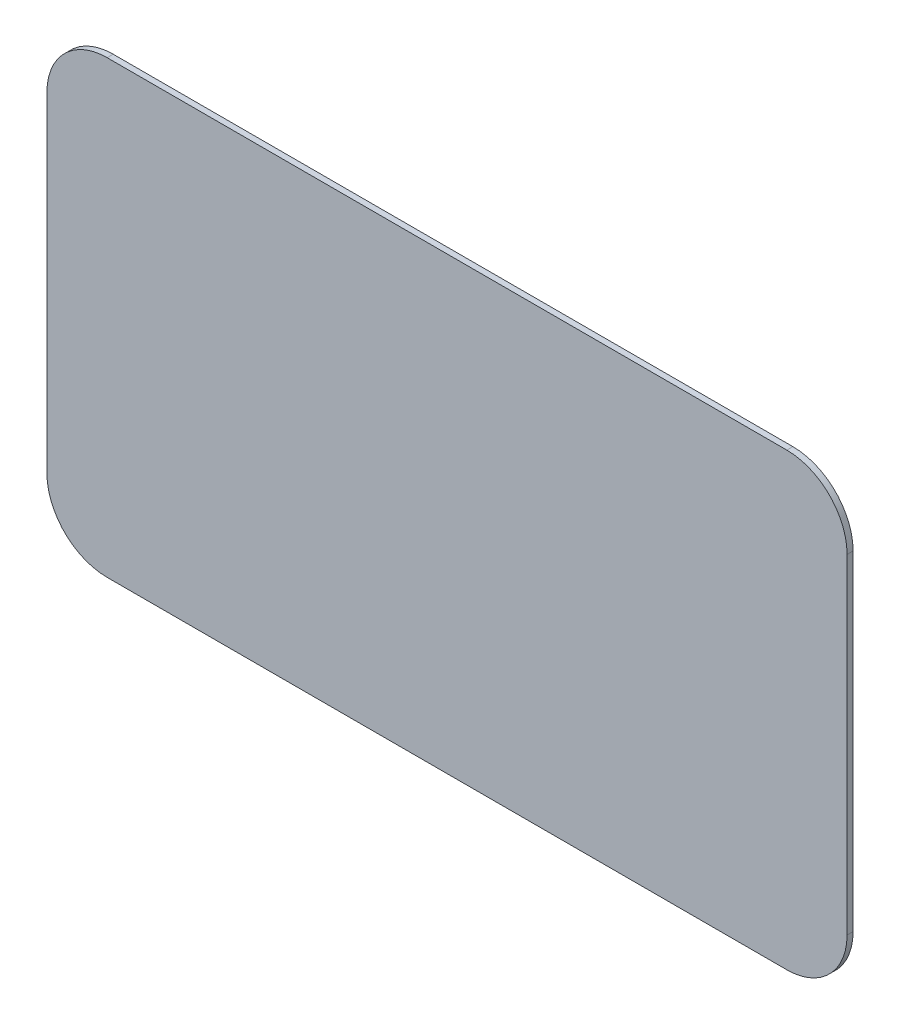
from build123d import *

# Parameters (mm, degrees)
SKETCH1_W           = 132.8
SKETCH1_H           = 74.7
BOSS_EXTRUDE1_DEPTH = 1
FILLET1_R           = 10


with BuildPart() as part:
    # Sketch1 → Boss-Extrude1 (new body)
    with BuildSketch(Plane.XY):
        Rectangle(SKETCH1_W, SKETCH1_H)
    extrude(amount=BOSS_EXTRUDE1_DEPTH)

    # Fillet1
    fillet1_edges = [part.edges().sort_by_distance(p)[0] for p in [
        (-66.4, -37.35, 0.5),
        (66.4, -37.35, 0.5),
        (66.4, 37.35, 0.5),
        (-66.4, 37.35, 0.5),
    ]]
    fillet(fillet1_edges, radius=FILLET1_R)


solid = part.part
